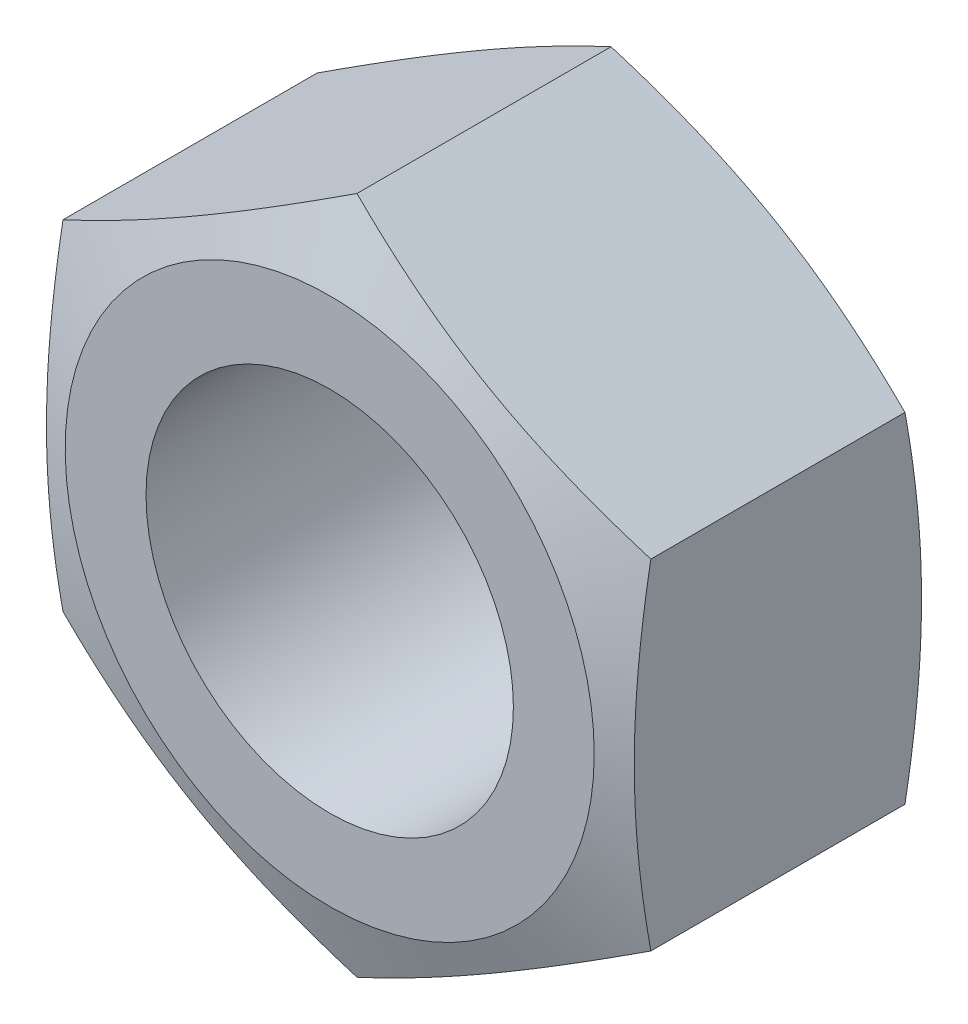
from build123d import *

# Parameters (mm, degrees)
BOSS_EXTRUDE1_DEPTH = 8.4
SKETCH5_R           = 5
CUT_EXTRUDE1_DEPTH  = 15.828800806


with BuildPart() as part:
    # Sketch1 → Boss-Extrude1 (new body)
    with BuildSketch(Plane.XY):
        Polygon((0, 9.237604307), (-8, 4.618802154), (-8, -4.618802154), (0, -9.237604307), (8, -4.618802154), (8, 4.618802154), align=None)
    extrude(amount=BOSS_EXTRUDE1_DEPTH)

    # Sketch4 → Cut-Revolve1 (revolve, cut)
    with BuildSketch(Plane(origin=(0, 0, 0), x_dir=(0, 0, -1), z_dir=(1, 0, 0)), mode=Mode.PRIVATE) as cut_revolve1_sk:
        Polygon((-8.4, -7.2), (-7.658372683, -9.237604307), (-8.4, -9.237604307), align=None)
    cut_revolve1 = revolve(cut_revolve1_sk.sketch.rotate(Axis((0, 0, 8.4), (0, 0, -1)), 119.999999987), axis=Axis((0, 0, 8.4), (0, 0, -1)), mode=Mode.SUBTRACT)

    # Mirror1: Cut-Revolve1 across plane
    add(cut_revolve1.mirror(Plane.XY.offset(4.2)), mode=Mode.SUBTRACT)

    # Sketch5 → Cut-Extrude1 (cut, through all)
    with BuildSketch(Plane.XY.offset(8.4)):
        Circle(SKETCH5_R)
    extrude(amount=-CUT_EXTRUDE1_DEPTH, mode=Mode.SUBTRACT)


solid = part.part
